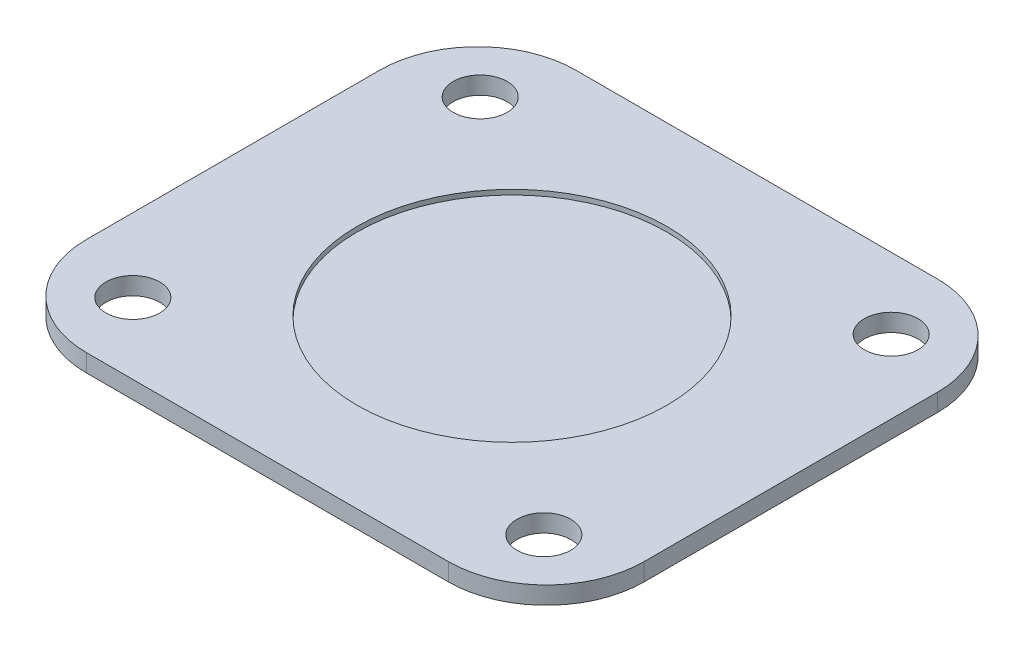
from build123d import *

# Parameters (mm, degrees)
BOSS_EXTRUDE1_DEPTH = 3.6
SKETCH2_R           = 31.666666667
CUT_EXTRUDE1_DEPTH  = 1
SKETCH4_R           = 5.5
CUT_EXTRUDE2_DEPTH  = 78.385241649


with BuildPart() as part:
    # Sketch1 → Boss-Extrude1 (new body)
    with BuildSketch(Plane(origin=(0, 0, 0), x_dir=(1, 0, 0), z_dir=(0, 1, 0))):
        with BuildLine():
            Line((-37, 50), (37, 50))
            ThreePointArc((37, 50), (51.142135624, 44.142135624), (57, 30))
            Line((57, 30), (57, -30))
            ThreePointArc((57, -30), (51.142135624, -44.142135624), (37, -50))
            Line((37, -50), (-37, -50))
            ThreePointArc((-37, -50), (-51.142135624, -44.142135624), (-57, -30))
            Line((-57, -30), (-57, 30))
            ThreePointArc((-57, 30), (-51.142135624, 44.142135624), (-37, 50))
        make_face()
    extrude(amount=-BOSS_EXTRUDE1_DEPTH)

    # Sketch2 → Cut-Extrude1 (cut)
    with BuildSketch(Plane(origin=(0, 0, 0), x_dir=(1, 0, 0), z_dir=(0, 1, 0))):
        with Locations(Location((0, 0, 0), (0, 0, 270))):
            Circle(SKETCH2_R)
    extrude(amount=-CUT_EXTRUDE1_DEPTH, mode=Mode.SUBTRACT)

    # Sketch3 → Revolve1 (revolve)
    with BuildSketch(Plane.XY, mode=Mode.PRIVATE) as revolve1_sk:
        with BuildLine():
            Line((0, -3.6), (38, -3.6))
            Line((38, -3.6), (31.599978616, -14.488457433))
            ThreePointArc((31.599978616, -14.488457433), (30.869015975, -15.210931287), (29.875767483, -15.475))
            Line((29.875767483, -15.475), (0, -15.475))
            Line((0, -15.475), (0, -3.6))
        make_face()
    revolve(revolve1_sk.sketch.rotate(Axis((0, -15.475, 0), (0, 1, 0)), 270), axis=Axis((0, -15.475, 0), (0, 1, 0)))

    # Sketch4 → Cut-Extrude2 (cut, through all)
    with BuildSketch(Plane(origin=(0, 0, 0), x_dir=(1, 0, 0), z_dir=(0, 1, 0))):
        with Locations(Location((-42, 35.5, 0), (0, 0, 270))):
            Circle(SKETCH4_R)
        with Locations(Location((42, 35.5, 0), (0, 0, 270))):
            Circle(SKETCH4_R)
        with Locations(Location((42, -35.5, 0), (0, 0, 270))):
            Circle(SKETCH4_R)
        with Locations(Location((-42, -35.5, 0), (0, 0, 270))):
            Circle(SKETCH4_R)
    extrude(amount=-CUT_EXTRUDE2_DEPTH, mode=Mode.SUBTRACT)


solid = part.part
